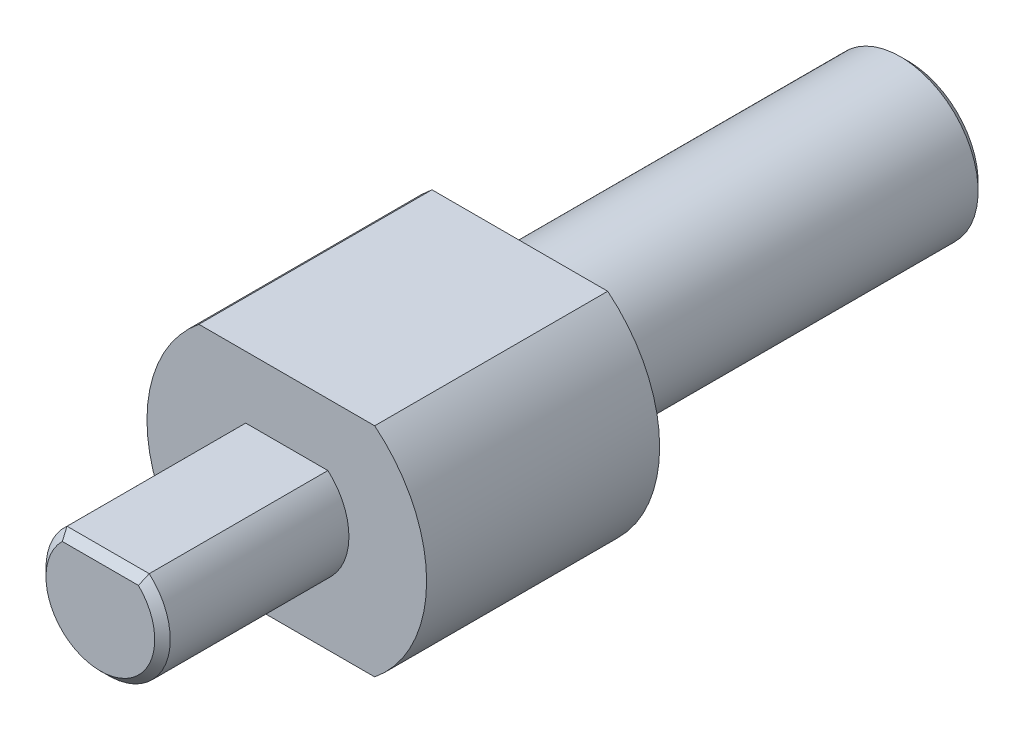
from build123d import *

# Parameters (mm, degrees)
BOSS_EXTRUDE1_DEPTH = 12
BOSS_EXTRUDE2_DEPTH = 15
SKETCH3_R           = 5
BOSS_EXTRUDE3_DEPTH = 25
CHAMFER1_SIZE       = 0.5


with BuildPart() as part:
    # Sketch1 → Boss-Extrude1 (new body)
    with BuildSketch(Plane.XY):
        with BuildLine():
            Line((2.645751311, 3), (-2.645751311, 3))
            ThreePointArc((-2.645751311, 3), (-1.645751311, -3.645751311), (4, 0))
            ThreePointArc((4, 0), (3.645751311, 1.645751311), (2.645751311, 3))
        make_face()
    extrude(amount=-BOSS_EXTRUDE1_DEPTH)

    # Sketch2 → Boss-Extrude2 (add)
    # profile 1 of 2: a face of its own
    with BuildSketch(Plane(origin=(0, 0, -12), x_dir=(-1, 0, 0), z_dir=(0, 0, -1))):
        with BuildLine():
            Line((5.656854249, 7), (-5.656854249, 7))
            ThreePointArc((-5.656854249, 7), (-9, 0), (-5.656854249, -7))
            Line((-5.656854249, -7), (5.656854249, -7))
            ThreePointArc((5.656854249, -7), (8.121320344, -3.878679656), (9, 0))
            ThreePointArc((9, 0), (8.121320344, 3.878679656), (5.656854249, 7))
        make_face()
        with BuildLine():
            ThreePointArc((2.645751311, 3), (0, -4), (-2.645751311, 3))
            Line((-2.645751311, 3), (2.645751311, 3))
        make_face(mode=Mode.SUBTRACT)
    # profile 2 of 2: a face of its own
    with BuildSketch(Plane(origin=(0, 0, -12), x_dir=(-1, 0, 0), z_dir=(0, 0, -1))):
        with BuildLine():
            Line((2.645751311, 3), (-2.645751311, 3))
            ThreePointArc((-2.645751311, 3), (0, -4), (2.645751311, 3))
        make_face()
    extrude(amount=BOSS_EXTRUDE2_DEPTH)

    # Sketch3 → Boss-Extrude3 (add)
    with BuildSketch(Plane(origin=(0, 0, -27), x_dir=(-1, 0, 0), z_dir=(0, 0, -1))):
        Circle(SKETCH3_R)
    extrude(amount=BOSS_EXTRUDE3_DEPTH)

    # Chamfer1
    chamfer1_edges = [part.edges().sort_by_distance(p)[0] for p in [
        (5, 0, -52),
        (0, 3, 0),
        (0, -4, 0),
    ]]
    chamfer(chamfer1_edges, length=CHAMFER1_SIZE)


solid = part.part
